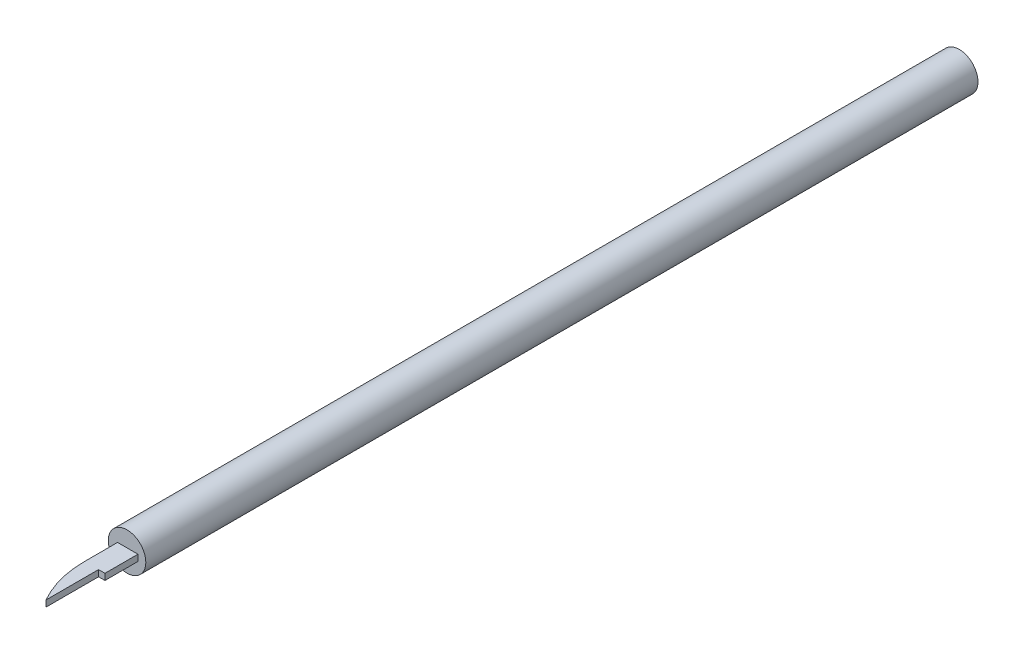
SolidWorks part; units mm, degrees
ref_plane "Front Plane" through (0, 0, 0) normal (0, 0, 1) x (1, 0, 0)
ref_plane "Top Plane" through (0, 0, 0) normal (0, 1, 0) x (1, 0, 0)
ref_plane "Right Plane" through (0, 0, 0) normal (1, 0, 0) x (0, 0, -1)
sketch "Sketch1" plane through (0, 0, 0) normal (0, 0, 1) x (1, 0, 0)
  circle A0 centre (0, 0) radius 1.5 construction
  circle A1 centre (0, 0) radius 1.5
extrude "Boss-Extrude1" add sketch "Sketch1" along normal blind 20 and the other way blind 46
sketch "Sketch2" plane through (0, 0, 20) normal (0, 0, 1) x (1, 0, 0)
  line L0 (-2.5, 2.5) -> (2.5, 2.5) construction
  line L1 (-2.5, 2.5) -> (-2.5, -2.5) construction
  line L2 (2.5, 2.5) -> (2.5, -2.5) construction
  line L3 (-2.5, -2.5) -> (2.5, -2.5) construction
  line L4 (-2.5, 2.5) -> (2.5, -2.5) construction
  line L5 (2.5, 2.5) -> (-2.5, -2.5) construction
  line L6 (40, 12) -> (-40, 12) construction
  circle A0 centre (0, 0) radius 1.5
  point P1 (0, 0)
  dimension "D3" = 3
  dimension "D1" = 5
  dimension "D2" = 5
extrude "Boss-Extrude2" add sketch "Sketch2" along normal blind 0.5
ref_plane "Plane4" through (0, 0, 0) normal (0, 1, 0) x (1, 0, 0)
sketch "Sketch3" plane through (0, 0, 0) normal (0, 1, 0) x (1, 0, 0)
  line L0 (0.8739, -20.5) -> (-0.7579, -20.5)
  line L9 (-0.7579, -20.5) -> (-0.7579, -23.1389)
  line L11 (0.3626, -27.3377) -> (0.3626, -23.1389)
  line L12 (0.3626, -23.1389) -> (0.8739, -23.1389)
  line L13 (0.8739, -23.1389) -> (0.8739, -20.5)
  line L14 (-1.5, -20.5) -> (1.5, -20.5) construction
  arc A1 (-0.7579, -23.1389) -> (0.3626, -27.3377) centre (7.6696, -23.1389) ccw
extrude "Boss-Extrude3" add sketch "Sketch3" along normal mid plane 0.5
